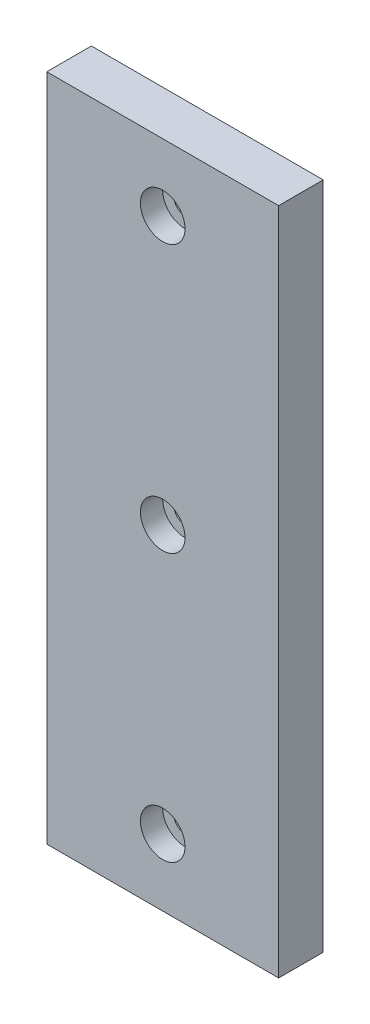
from build123d import *

# Parameters (mm, degrees)
SKETCH1_W           = 52
SKETCH1_H           = 150
BOSS_EXTRUDE1_DEPTH = 5
HOLE1_D             = 5
HOLE1_CBORE_D       = 10
HOLE1_CBORE_DEPTH   = 5


with BuildPart() as part:
    # Sketch1 → Boss-Extrude1 (new, symmetric)
    with BuildSketch(Plane.XY):
        Rectangle(SKETCH1_W, SKETCH1_H)
    extrude(amount=BOSS_EXTRUDE1_DEPTH, both=True)

    # Hole1 (through all)
    with Locations(Plane.XY.offset(5)):
        with Locations((0, 60), (0, -60), (0, 0)):
            CounterBoreHole(HOLE1_D / 2, HOLE1_CBORE_D / 2, HOLE1_CBORE_DEPTH)


solid = part.part
